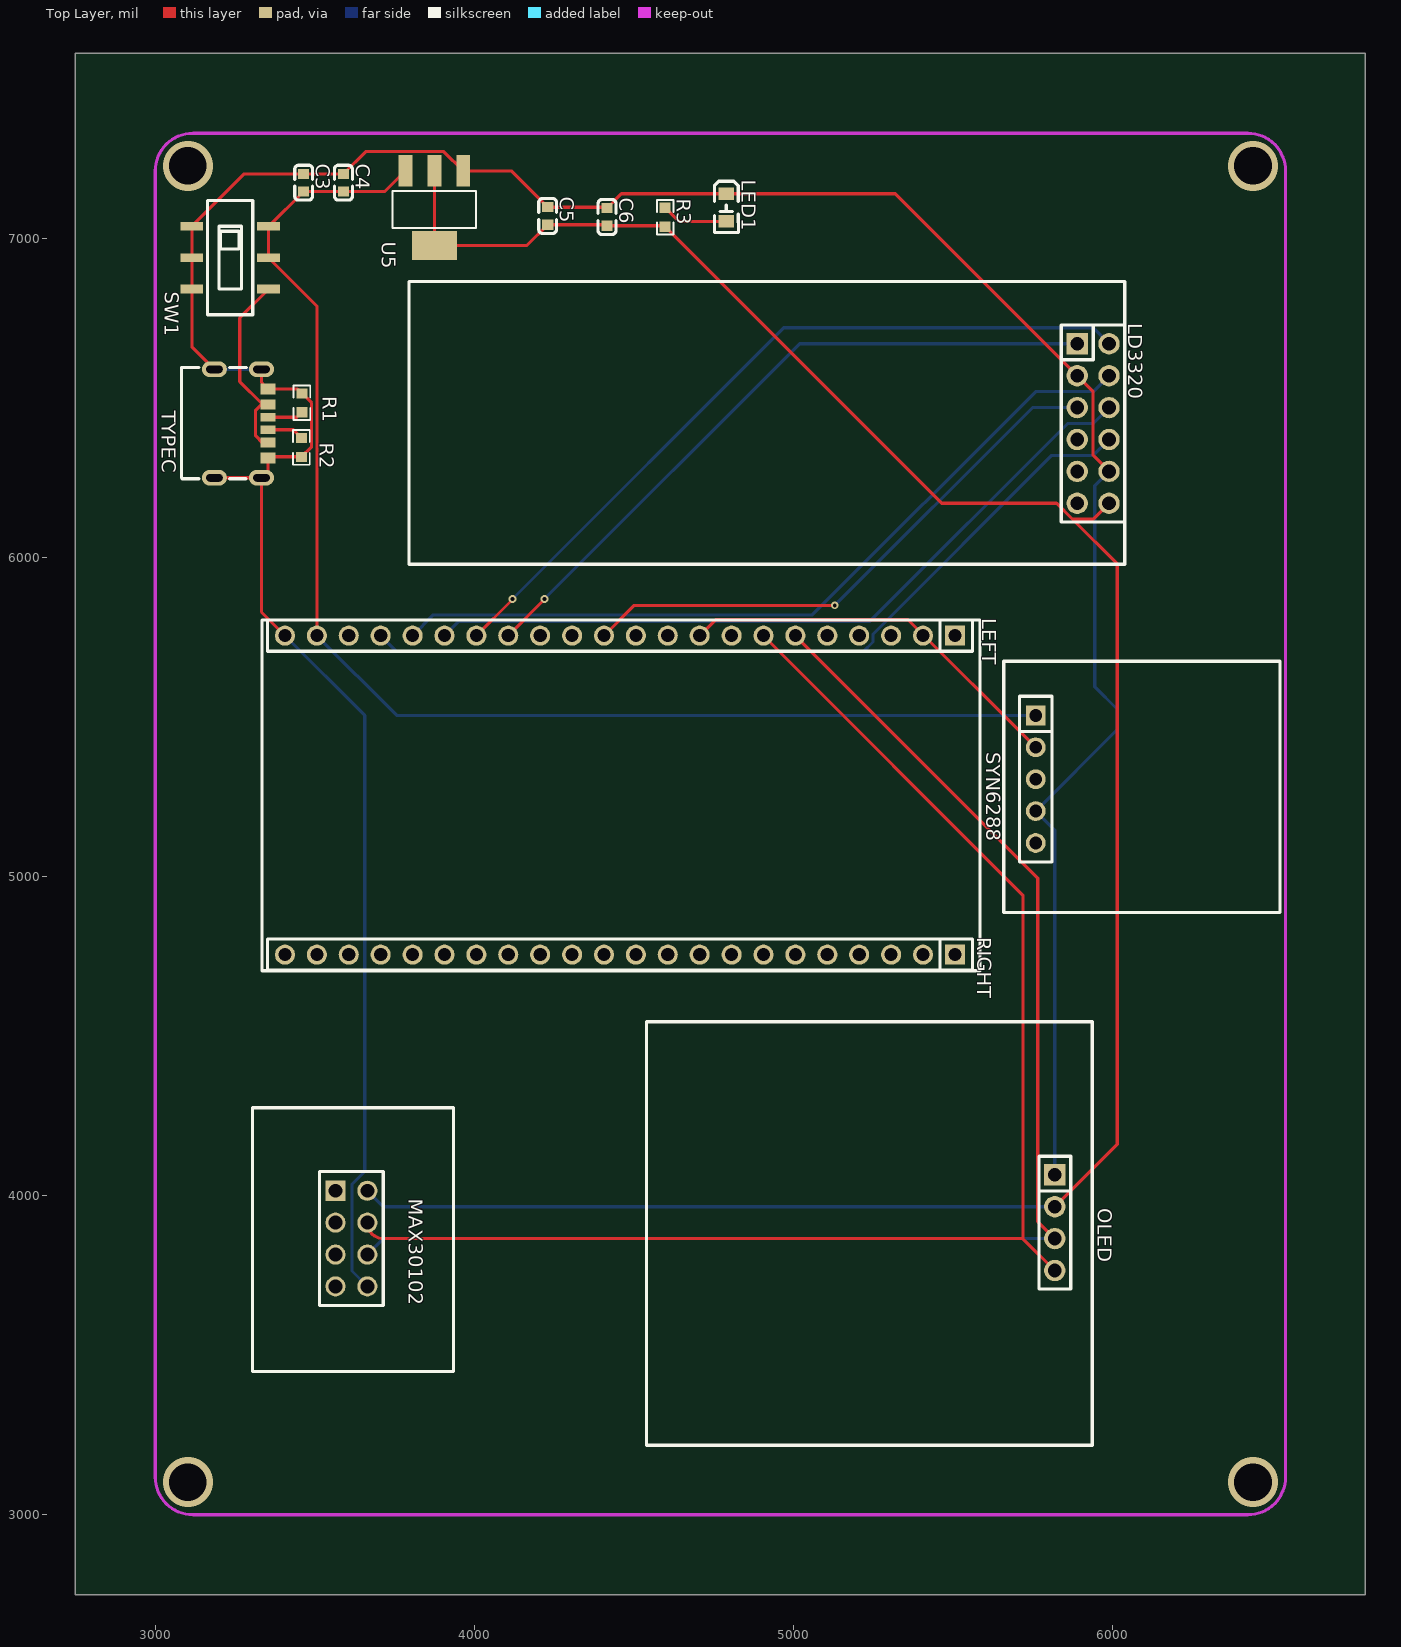
[diagram p0: Top Layer view]
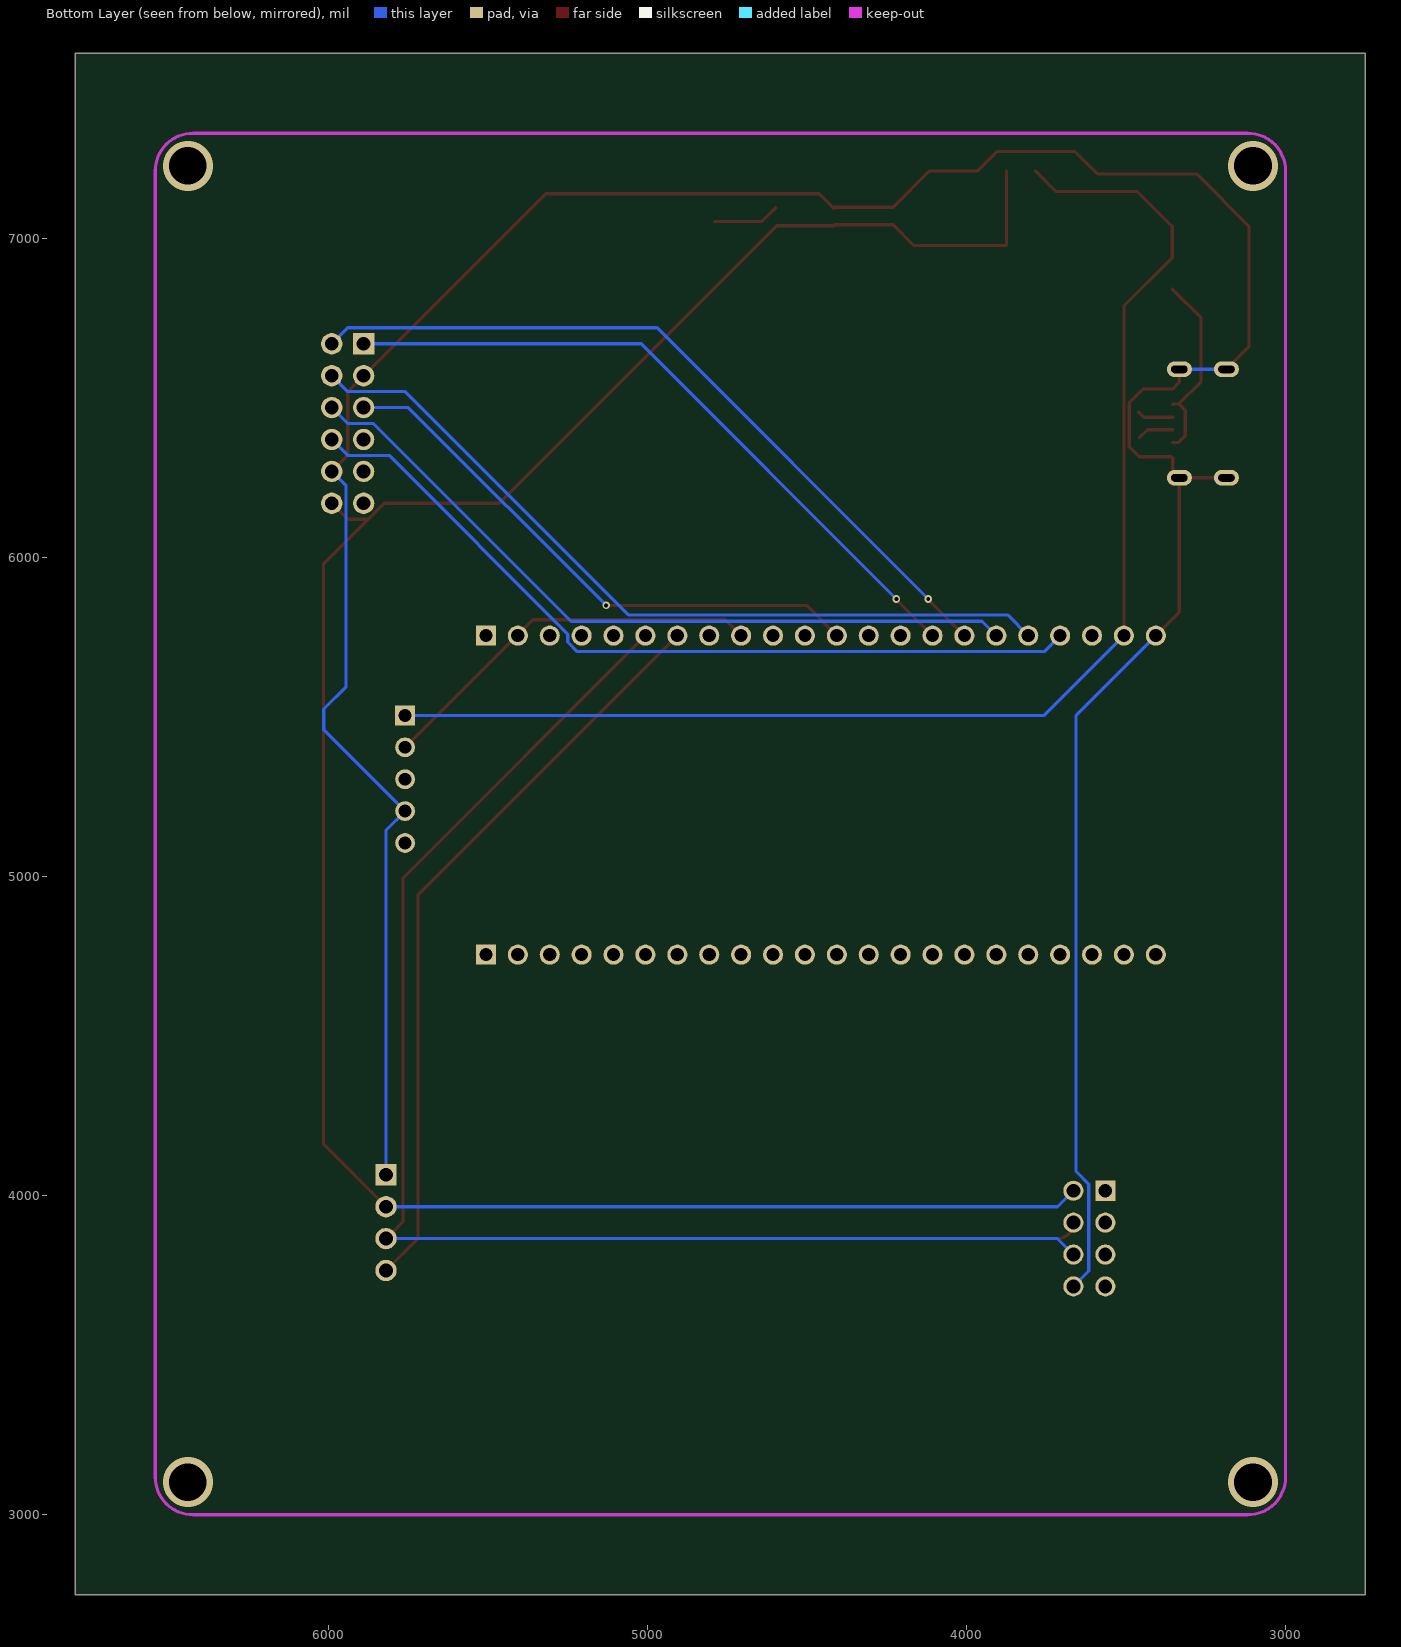
[diagram p1: Bottom Layer view, seen from below]
# Altium PCB MISC49905.pcbdoc
Units mil, origin at the board's own origin, x right, y up, seen from the top; angles counter-clockwise.
Board outline 4043.31 x 4830.71 mil, 2 copper layers (Top Layer, Bottom Layer), stack 62.206 mil thick; 17 components, 17 nets, 109 pads, 7 vias.

## Layer stack, top to bottom
Top Solder Mask Layer: solder mask 0.394, Dk 3.3
Top Layer: signal copper 1.379
Dielectric1: surface 59.449, FR4, Dk 4.5
Bottom Layer: signal copper 1.378
Bottom Solder Mask Layer: solder mask 0.394, Dk 3.3

## Board outline
6793.31,2750 2750,2750 2750,7580.71 6793.31,7580.71

## Design rules (kind name [scope] priority, off if disabled: settings)
BoardOutlineClearance copperThickness2oz_1 [All] p2 off: genericclearance=7.99 ignorepadtopadclearanceinfootprint=FALSE except(0: Arc-SplitContinuation Track-SplitContinuation SMDPad-SplitContinuation THPad-SplitContinuation Via-SplitContinuation Fill-SplitContinuation Region-SplitContinuation Poly-SplitContinuation Text-SplitContinuation Hole-SplitContinuation; 5.98: Arc-CutoutEdge SMDPad-CutoutEdge THPad-CutoutEdge Via-CutoutEdge Fill-CutoutEdge Region-CutoutEdge Text-CutoutEdge; 6.93: Hole-OutlineEdge Hole-CutoutEdge; 10: Poly-OutlineEdge Poly-CutoutEdge; 11.81: Arc-OutlineEdge Track-OutlineEdge SMDPad-OutlineEdge THPad-OutlineEdge Via-OutlineEdge Fill-OutlineEdge Region-OutlineEdge Text-OutlineEdge Track-CutoutEdge)
BoardOutlineClearance copperThickness1oz_1 [All] p4: genericclearance=4.02 ignorepadtopadclearanceinfootprint=FALSE except(0: Arc-SplitContinuation Track-SplitContinuation SMDPad-SplitContinuation THPad-SplitContinuation Via-SplitContinuation Fill-SplitContinuation Region-SplitContinuation Poly-SplitContinuation Text-SplitContinuation Hole-SplitContinuation; 6: SMDPad-CutoutEdge THPad-CutoutEdge Via-CutoutEdge Fill-CutoutEdge Region-CutoutEdge Text-CutoutEdge; 6.93: Hole-OutlineEdge Hole-CutoutEdge; 10: Poly-OutlineEdge Poly-CutoutEdge; 11.8: Arc-OutlineEdge Track-OutlineEdge SMDPad-OutlineEdge THPad-OutlineEdge Via-OutlineEdge Fill-OutlineEdge Region-OutlineEdge Text-OutlineEdge; 11.81: Arc-CutoutEdge Track-CutoutEdge)
Clearance copperThickness2oz [All] p1 off: gap=7.99 ignorepadtopadclearanceinfootprint=FALSE except(5.98: SMDPad-Track SMDPad-SMDPad THPad-Track SMDPad-THPad THPad-THPad Track-Via SMDPad-Via THPad-Via Via-Via Fill-Track Region-Track Fill-SMDPad Region-SMDPad Fill-THPad Region-THPad Fill-Via Region-Via Fill-Fill Fill-Region Region-Region Arc-Track Arc-SMDPad Arc-THPad Arc-Via Fill-Arc Region-Arc Arc-Arc Text-Track SMDPad-Text Text-THPad Text-Via Fill-Text Region-Text Arc-Text Text-Text; 6.93: Hole-Track Hole-SMDPad Hole-THPad Hole-Via Fill-Hole Region-Hole Hole-Arc Hole-Text; 10: Poly-Track Poly-SMDPad Poly-THPad Poly-Via Poly-Fill Poly-Region Poly-Poly Poly-Arc Poly-Text Poly-Hole)
Clearance copperThickness1oz [All] p3: gap=4.02 ignorepadtopadclearanceinfootprint=FALSE except(5.98: SMDPad-Track SMDPad-SMDPad THPad-Track SMDPad-THPad THPad-THPad Track-Via SMDPad-Via THPad-Via Via-Via Fill-Track Region-Track Fill-SMDPad Region-SMDPad Fill-THPad Region-THPad Fill-Via Region-Via Fill-Fill Fill-Region Region-Region; 6: Arc-Track Arc-SMDPad Arc-THPad Arc-Via Fill-Arc Region-Arc Arc-Arc Text-Track SMDPad-Text Text-THPad Text-Via Fill-Text Region-Text Arc-Text Text-Text; 6.93: Hole-Track Hole-SMDPad Hole-THPad Hole-Via Fill-Hole Region-Hole Hole-Arc Hole-Text; 10: Poly-Track Poly-SMDPad Poly-THPad Poly-Via Poly-Fill Poly-Region Poly-Poly Poly-Arc Poly-Text Poly-Hole)
DiffPairsRouting differentialPair [All] p1: maxlimit=6 minlimit=6 mostfreqgap=6 toplayer_minwidth=5 toplayer_prefwidth=10 toplayer_maxwidth=100 toplayer_mingap=6 toplayer_prefgap=6 toplayer_maxgap=6 bottomlayer_minwidth=5 bottomlayer_prefwidth=10 bottomlayer_maxwidth=100 bottomlayer_mingap=6 bottomlayer_prefgap=6 bottomlayer_maxgap=6 maxuncoupledlength=10
HoleToHoleClearance otherClearance [All] p1: gap=11.81 allowstackedmicrovias=TRUE
Length netLength [All] p1: minlimit=0 maxlimit=0
MatchedLengths netLengthTolerance [All] p1: tolerance=1000
PasteMaskExpansion pasteMaskExpansion [All] p1: expansion=0
PlaneConnect innerPlane [All] p1: planeconnectstyle=Relief reliefexpansion=20 reliefentries=4 reliefconductorwidth=10 reliefairgap=10
PolygonConnect copperRegion [All] p1: connectstyle=Relief reliefconductorwidth=10 reliefentries=4 polygonreliefangle="90 Angle" airgapwidth=10 via.connectstyle=Relief via.reliefconductorwidth=10 via.reliefentries=4 via.polygonreliefangle="90 Angle" via.airgapwidth=10
RoutingVias viaSize [All] p1: holewidth=12.01 width=24.02 viastyle="Through Hole" minholewidth=11.81 minwidth=19.68 maxholewidth=248.03 maxwidth=393.7
SolderMaskExpansion solderMaskExpansion [IsVia] p1: expansion=-1000 istentingtop=TRUE
SolderMaskExpansion solderMaskExpansion [All] p2: expansion=2 istentingtop=FALSE
Width copperThickness2oz_2 [All] p1 off: maxlimit=100 minlimit=8 preferedwidth=10
Width copperThickness1oz_2 [All] p2: maxlimit=100 minlimit=5 preferedwidth=10

## Components (designator, comment, footprint, x,y, rotation, side; value= is the part's Value field where it differs from the comment)
C3 "10uF" C0603 3465,7175.71 r270 top
C4 "100nF" C0603 3590,7175.71 r270 top
C5 "100nf" C0603 4230,7071.36 r270 top
C6 "10uf" C0603 4416.22,7068.28 r270 top
LD3320 "ZX-PM2.54-2-6PY" HDR-TH_12P-P2.54-V-F-R2-C6-S2.54 5940,6420.71 r270 top
LED1 "" LED_0805 4790,7095.71 r270 top
LEFT "ZX-PM2.54-1-22PY" HDR-TH_22P-P2.54-V-F 4456.69,5755.91 r180 top locked
MAX30102 "ZX-PM2.54-2-4PY" HDR-TH_8P-P2.54-V-F-R2-C4-S2.54 3615,3865.71 r270 top
OLED "ZX-PM2.54-1-4PY" HDR-TH_4P-P2.54-V-F 5820,3915.71 r270 top
R1 "5.1K" R0603 3460,6485.71 r90 top
R2 "5.1K" R0603 3458.23,6345.96 r270 top
R3 "1K" R0603 4598.48,7067.38 r90 top
RIGHT "ZX-PM2.54-1-22PY" HDR-TH_22P-P2.54-V-F 4456.69,4755.91 r180 top locked
SW1 "SS-3235S-L1" SW-SMD_SS-3235S-LX 3235,6940.71 r90 top
SYN6288 "ZX-PM2.54-1-5PY" HDR-TH_5P-P2.54-V-F-B 5760,5305.71 r270 top
TYPEC "" "USB_ TYPE-C-6P" 3269.62,6425.71 r270 top
U5 "AMS1117-3.3" SOT-223-3_L6.5-W3.4-P2.30-LS7.0-BR 3875,7095.71 r90 top

## Footprints (in the part's own frame and the unit in brackets; to place one, negate y for a bottom-side part, rotate by r counter-clockwise, add the part's x,y. Pads: shape width x height; smd on the part's side, far side on the other; paste and mask are expansions set on the pad)
C0603 [mm]
  rect 0.8x0.9 smd: 1(-0.7,0) 2(0.7,0)
  silkscreen extent -1.39,-0.71 1.39,0.71
HDR-TH_4P-P2.54-V-F [mm]
  rect 1.7x1.7 hole 1.1: 1(-3.81,0)
  round 1.7 hole 1.1: 2(-1.27,0) 3(1.27,0) 4(3.81,0)
  silkscreen extent -5.29,-1.27 5.29,1.27
HDR-TH_5P-P2.54-V-F-B [mil]
  rect 62x62 hole 40.16: 1(-200,0)
  round 62 hole 40.16: 2(-100,0) 3(0,0) 4(100,0) 5(200,0)
  silkscreen extent -260,-51 260,51
HDR-TH_8P-P2.54-V-F-R2-C4-S2.54 [mm]
  rect 1.6x1.6 hole 1.1: 1(-3.81,-1.27)
  round 1.6 hole 1.1: 2(-3.81,1.27) 3(-1.27,-1.27) 4(-1.27,1.27) 5(1.27,-1.27) 6(1.27,1.27) 7(3.81,-1.27) 8(3.81,1.27)
  silkscreen extent -5.33,-2.54 5.33,2.54
HDR-TH_12P-P2.54-V-F-R2-C6-S2.54 [mm]
  rect 1.7x1.7 hole 1.1: 1(-6.35,-1.27)
  round 1.7 hole 1.1: 2(-6.35,1.27) 3(-3.81,-1.27) 4(-3.81,1.27) 5(-1.27,-1.27) 6(-1.27,1.27) 7(1.27,-1.27) 8(1.27,1.27) 9(3.81,-1.27) 10(3.81,1.27) 11(6.35,-1.27) 12(6.35,1.27)
  silkscreen extent -7.85,-2.54 7.85,2.54
HDR-TH_22P-P2.54-V-F [mm]
  rect 1.6x1.6 hole 1.05: 1(-26.67,0)
  round 1.6 hole 1.05: 2(-24.13,0) 3(-21.59,0) 4(-19.05,0) 5(-16.51,0) 6(-13.97,0) 7(-11.43,0) 8(-8.89,0) 9(-6.35,0) 10(-3.81,0) 11(-1.27,0) 12(1.27,0) 13(3.81,0) 14(6.35,0) 15(8.89,0) 16(11.43,0) 17(13.97,0) 18(16.51,0) 19(19.05,0) 20(21.59,0) 21(24.13,0) 22(26.67,0)
  silkscreen extent -28.06,-1.25 28.06,1.25
LED_0805 [mm]
  rect 1x1.25 smd paste+0 mask+0.051: 1(-1.15,0.005) 2(1.05,0.005)
  silkscreen extent -2.15,-0.94 1.93,0.97
R0603 [mil]
  rect 31.75x34.02 smd paste-3937.01 mask+2: 1(-29.66,0) 2(29.66,0)
  silkscreen extent -55,-26 55,26
SOT-223-3_L6.5-W3.4-P2.30-LS7.0-BR [mm]
  rect 2.5x1.1 smd: 1(2.97,-2.3) 2(2.97,0) 3(2.97,2.3)
  rect 2.34x3.6 smd: 4(-2.97,0)
  silkscreen extent -1.57,-3.33 1.37,3.33
SW-SMD_SS-3235S-LX [mm]
  rect 0.7x1.8 smd: 1(-2.5,3.05) 2(0,3.05) 3(2.5,3.05) 4(-2.5,-3.05) 5(0,-3.05) 6(2.5,-3.05)
  silkscreen extent -4.55,-1.8 4.55,1.8
"USB_ TYPE-C-6P" [mm]
  oval 1.25x2 hole 0.6 slot 1.3 at 90 deg paste+0 mask+0.05: 7(-4.193,1.611) 8(4.447,1.611) 9(-4.193,-2.139) 10(4.447,-2.139)
  rect 0.7x1.2 smd paste-100 mask+0.05: A5(-0.373,2.139) B5(0.627,2.139)
  rect 0.8x1.2 smd paste-100 mask+0.05: A9(1.647,2.139) B9(-1.393,2.139)
  rect 0.9x1.2 smd paste-100 mask+0.05: A12(2.877,2.139) B12(-2.623,2.139)
  silkscreen extent -4.34,-4.75 4.52,0.39

## Via types
v1: diameter 157.48, hole 118.1, Top Layer to Bottom Layer, 4 vias
v2: diameter 24.02, hole 12, Top Layer to Bottom Layer, 3 vias

## Nets (pads, with @x,y where several pads share a name; then routed paths per layer and width w, separated by ;. In a path a pad name is that pad's centre, name@x,y a point inside that pad or via, vN(x,y) a via of type N, cw(c..) or ccw(c..) an arc to the next point about the centre after c; other vN are vias at no path point)
3.3v: C5.2 C6.2 LD3320.12 MAX30102.2 OLED.2 R3.1 U5.2 U5.4
3.3V:  | length 7248.5
  Top Layer w10: 3875,7212.64 3875,6978.78 4164.98,6978.78 4230,7043.8 4413.13,7043.8 4416.21,7040.72 4595.48,7040.72 4598.48,7037.72 5465.5,6170.71 5825.49,6170.71 5875.49,6120.71 ; 5820,3965.71 6015.49,4161.2 6015.49,5980.71 5875.49,6120.71 ; 5990,6170.71 5940,6120.71 5875.49,6120.71
  Bottom Layer w10: 3665,4015.71 3715,3965.71 5820,3965.71
$1N34: R1.1 TYPEC.A5 | length 112.6
  Top Layer w10: TYPEC.A5 3444.34,6440.39 R1.1
$1N35: R2.1 TYPEC.B5 | length 114.9
  Top Layer w10: TYPEC.B5 3432.83,6401.02 R2.1
$1N43: LED1.2 R3.2 | length 209.4
  Top Layer w10: R3.2 4641.16,7054.37 LED1.2
+5V: C3.2 C4.2 LEFT.21 SW1.5 SW1.6 SYN6288.1 U5.3 | length 4204.2
  Top Layer w10: LEFT.21 3506.7,6789.1 SW1.5 SW1.6 3355.98,7039.13 3465,7148.15 3590,7148.15 3719.96,7148.15 U5.3
  Bottom Layer w10: LEFT.21 3756.89,5505.71 SYN6288.1
GND: C3.1 C4.1 C5.1 C6.1 LD3320.3 LD3320.10 LED1.1 LEFT.22 MAX30102.8 OLED.1 R1.2 R2.2 SW1.1 SW1.2 SW1.3 SYN6288.4 TYPEC.7 TYPEC.8 TYPEC.9 TYPEC.10 TYPEC.A12 TYPEC.B12 U5.1 | length 9986.7
  Top Layer w10: TYPEC.10 TYPEC.8 ; TYPEC.9 3114.92,6661.28 SW1.1 SW1.2 SW1.3 3279.05,7203.27 C3.1 C4.1 3660,7273.27 3904.92,7273.27 3965.55,7212.64 4116.29,7212.64 C5.1 4413.13,7098.92 C6.1 4461.36,7140.99 LED1.1 5319.72,7140.99 LD3320.3 5940,6520.71 5940,6320.71 LD3320.10 ; TYPEC.7 3333.05,6549.77 TYPEC.B12 3446.39,6528.98 R1.2 3490,6485.37 3490,6348.07 R2.2 3357.7,6316.3 TYPEC.A12 3353.84,6271.42 TYPEC.8 ; LEFT.22 3333.05,5829.55 TYPEC.8
  Bottom Layer w10: TYPEC.9 TYPEC.7 ; LEFT.22 3656.69,5505.91 3656.69,4075.91 3616.69,4035.91 3616.69,3764.01 MAX30102.8 ; OLED.1 5820,5145.71 SYN6288.4 6015,5460.71 6015,5525.72 5945,5595.72 5945,6225.71 LD3320.10
IO6: LEFT.6 MAX30102.6 OLED.3 | length 4402.8
  Top Layer w10: LEFT.6 5766.69,4995.91 5766.69,3919.01 OLED.3
  Bottom Layer w10: MAX30102.6 3715,3865.71 OLED.3
IO7: LEFT.7 MAX30102.4 OLED.4 | length 4452
  Top Layer w10: MAX30102.4 ccw(c3715,3915.71) 3715,3865.71 5720,3865.71 ; LEFT.7 5720,4942.6 5720,3865.71 ; OLED.4 5720,3865.71
IO8: LD3320.5 LEFT.12 | length 1779.4
  Top Layer w10: LEFT.12 4501.5,5850.71 v2(5130,5850.71)
  Bottom Layer w10: v2(5130,5850.71) 5750,6470.71 LD3320.5
IO9: LD3320.1 LEFT.15 | length 2163.1
  Top Layer w10: LEFT.15 4220,5869.21 v2(4220,5870.71)
  Bottom Layer w10: v2(4220,5870.71) 5020,6670.71 LD3320.1
IO10: LD3320.2 LEFT.16 | length 2404.5
  Top Layer w10: LEFT.16 4120,5869.21 v2(4120,5870.71)
  Bottom Layer w10: v2(4120,5870.71) 4970,6720.71 5940,6720.71 LD3320.2
IO11: LD3320.6 LEFT.17 | length 2379.4
  Bottom Layer w10: LEFT.17 3951.5,5800.71 5240,5800.71 5860,6420.71 5940,6420.71 LD3320.6
IO12: LD3320.4 LEFT.18 | length 2520.8
  Bottom Layer w10: LEFT.18 3871.5,5820.71 5060,5820.71 5760,6520.71 5940,6520.71 LD3320.4
IO13: LD3320.8 LEFT.19 | length 2593.9
  Bottom Layer w10: LEFT.19 3756.7,5705.9 5220,5705.9 5250,5735.9 5250,5760.71 5810,6320.71 5940,6320.71 LD3320.8
IO16: LEFT.9 SYN6288.2 | length 1239.8
  Top Layer w10: LEFT.9 4756.69,5805.9 5359.81,5805.9 SYN6288.2
VCC+5V: SW1.4 TYPEC.A9 TYPEC.B9 | length 602.7
  Top Layer w10: TYPEC.A9 3336.06,6360.87 3314.65,6382.29 3314.65,6462.29 TYPEC.B9@3334.65,6482.29 ; TYPEC.B9 3352.1,6482.29 TYPEC.B9@3334.65,6482.29 ; SW1.4 3264.65,6751.85 3264.65,6552.29 TYPEC.B9@3334.65,6482.29
pads on no net: LD3320.7 LD3320.9 LD3320.11 LEFT.1 LEFT.2 LEFT.3 LEFT.4 LEFT.5 LEFT.8 LEFT.10 LEFT.11 LEFT.13 LEFT.14 LEFT.20 MAX30102.1 MAX30102.3 MAX30102.5 MAX30102.7 RIGHT.1 RIGHT.2 RIGHT.3 RIGHT.4 RIGHT.5 RIGHT.6 RIGHT.7 RIGHT.8 RIGHT.9 RIGHT.10 RIGHT.11 RIGHT.12 RIGHT.13 RIGHT.14 RIGHT.15 RIGHT.16 RIGHT.17 RIGHT.18 RIGHT.19 RIGHT.20 RIGHT.21 RIGHT.22 SYN6288.3 SYN6288.5
copper on no net:
  other v1: 3102.36,3102.36 6440.94,3102.36 3102.36,7228.35 6440.94,7228.35

## Keep-outs
Board Outline Layer:
  lines w10: 3000,3118.11 3000,7212.6 cw(c3118.11,7212.6) 3118.11,7330.71 6425.2,7330.71 cw(c6425.2,7212.6) 6543.31,7212.6 6543.31,3118.11 cw(c6425.2,3118.11) 6425.2,3000 3118.11,3000 cw(c3118.11,3118.11) 3000,3118.11

## Silkscreen, mask and mechanical layers (free items; w line width, h text height)
Top Silkscreen Layer:
  lines w10: 3305,3448.94 3305,4275.71 3934.92,4275.71 3934.92,3448.94 3305,3448.94 ; 3335,4705.12 3335,5805.12 5585,5805.12 5585,4705.12 3335,4705.12 ; 3795,5979.88 3795,6865.71 6039.09,6865.71 6039.09,5979.88 3795,5979.88 ; 4540,3217.76 4540,4545.71 5937.24,4545.71 5937.24,3217.76 4540,3217.76 ; 5660,4888.31 5660,5675.71 6526.14,5675.71 6526.14,4888.31 5660,4888.31